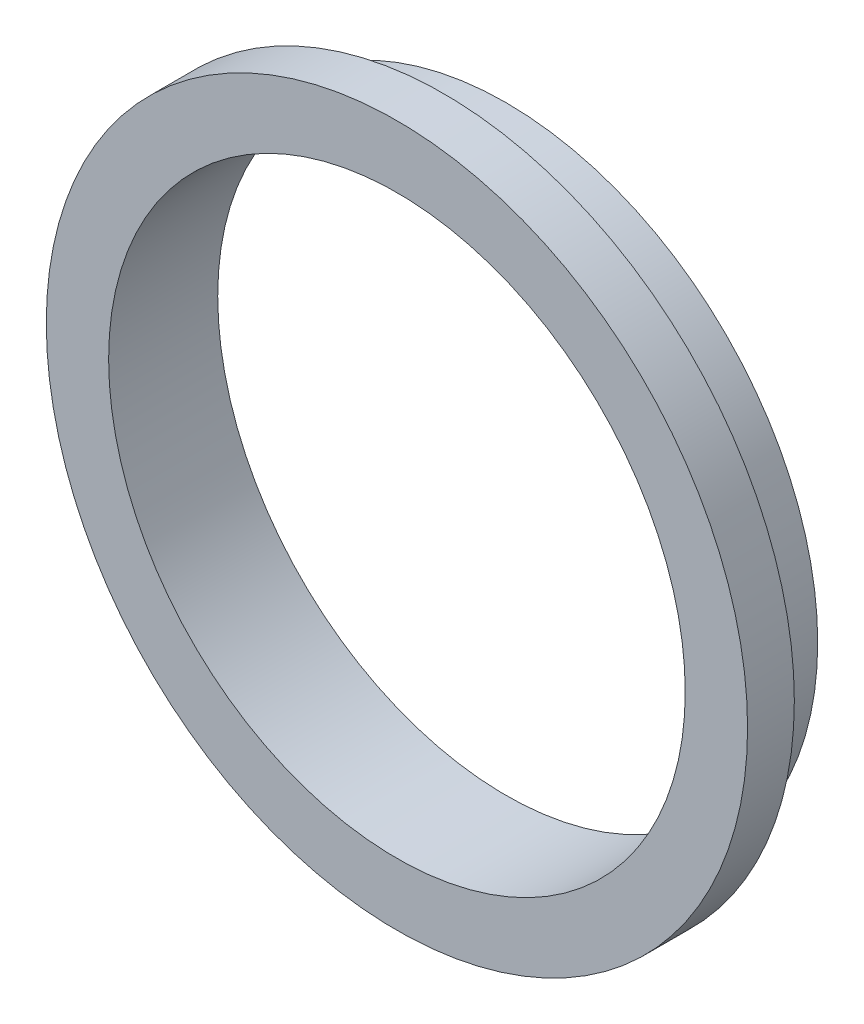
from build123d import *
from build123d.topology import SkipClean

# Parameters (mm, degrees)
SKETCH1_R           = 22.5
SKETCH1_R_2         = 18.5
BOSS_EXTRUDE1_DEPTH = 3
BOSS_EXTRUDE2_START = 4
SKETCH3_R           = 20
SKETCH3_R_2         = 18.5
BOSS_EXTRUDE2_DEPTH = 4


with BuildPart() as part:
    # Sketch1 → Boss-Extrude1 (new body)
    with BuildSketch(Plane.XY):
        Circle(SKETCH1_R)
        Circle(SKETCH1_R_2, mode=Mode.SUBTRACT)
    extrude(amount=BOSS_EXTRUDE1_DEPTH)

    # Sketch3 → Boss-Extrude2 (add)
    with SkipClean():  # the faces are left unmerged after this step: merging them gives an invalid solid
        with BuildSketch(Plane(origin=(0, 0, 0), x_dir=(-1, 0, 0), z_dir=(0, 0, -1)).offset(BOSS_EXTRUDE2_START)):
            with Locations(Location((0, 0, 0), (0, 0, 180))):
                Circle(SKETCH3_R)
            Circle(SKETCH3_R_2, mode=Mode.SUBTRACT)
        extrude(amount=-BOSS_EXTRUDE2_DEPTH)


solid = part.part
